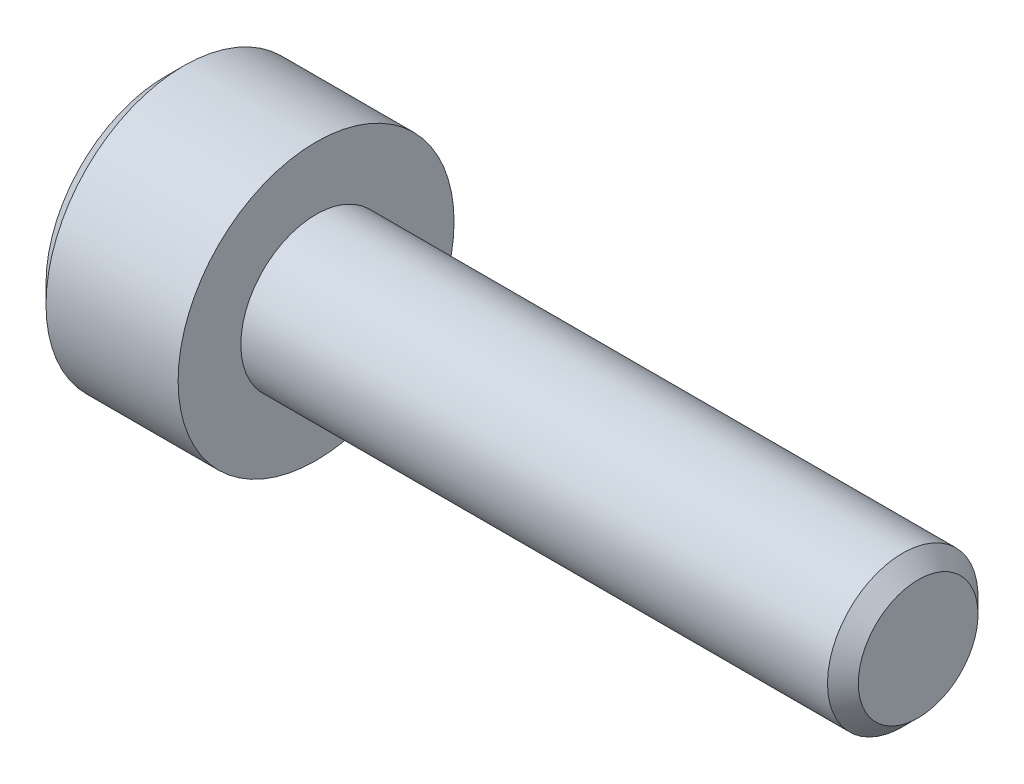
from build123d import *

# Parameters (mm, degrees)
CUT_EXTRUDE1_DEPTH = 1.5


with BuildPart() as part:
    # Sketch1 → Revolve1 (revolve)
    with BuildSketch(Plane.XY, mode=Mode.PRIVATE) as revolve1_sk:
        Polygon((-3, 0), (-3, 2.383333333), (-2.633333333, 2.75), (0, 2.75), (0, 1.5), (11.6928325, 1.5), (12, 1.1928325), (12, 0), align=None)
    revolve(revolve1_sk.sketch.rotate(Axis((12, 0, 0), (-1, 0, 0)), 270), axis=Axis((12, 0, 0), (-1, 0, 0)))

    # Sketch2 → Cut-Revolve1 (revolve, cut)
    with BuildSketch(Plane.XY, mode=Mode.PRIVATE) as cut_revolve1_sk:
        Polygon((-3, 0), (-3, 1.25), (-1.5, 1.25), (-1.165063509, 0), align=None)
    revolve(cut_revolve1_sk.sketch.rotate(Axis((-1.165063509, 0, 0), (-1, 0, 0)), 270), axis=Axis((-1.165063509, 0, 0), (-1, 0, 0)), mode=Mode.SUBTRACT)

    # Sketch3 → Cut-Extrude1 (cut)
    with BuildSketch(Plane(origin=(-3, 0, 0), x_dir=(0, 0, -1), z_dir=(1, 0, 0))):
        Polygon((-1.25, 0.721687836), (-1.25, -0.721687836), (0, -1.443375673), (1.25, -0.721687836), (1.25, 0.721687836), (0, 1.443375673), align=None)
    extrude(amount=CUT_EXTRUDE1_DEPTH, mode=Mode.SUBTRACT)


solid = part.part
